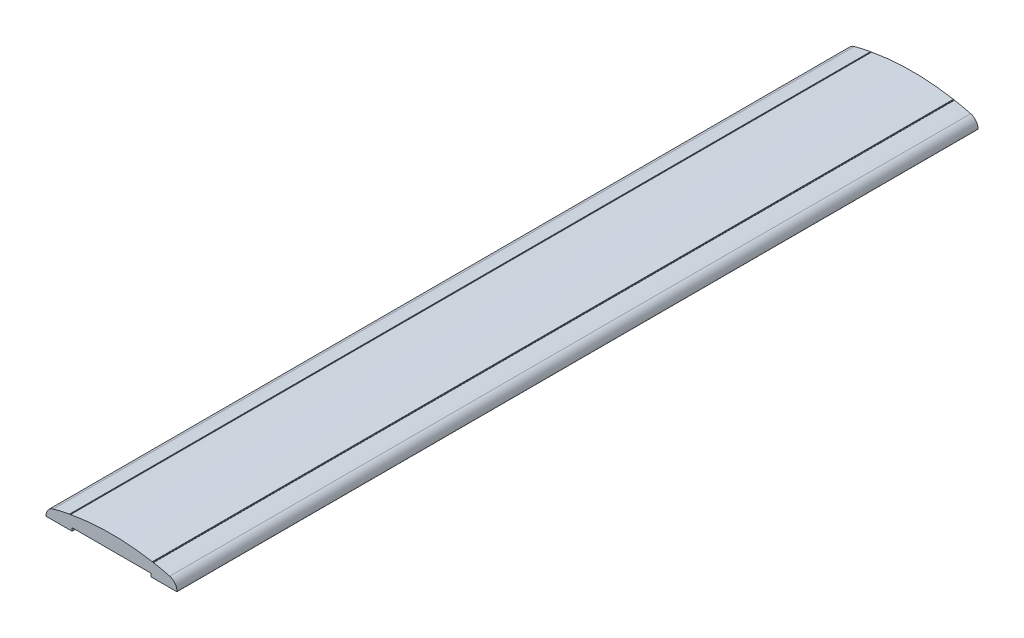
SolidWorks part; units mm, degrees
material "6063-T5"
ref_plane "前视基准面" through (0, 0, 0) normal (0, 0, 1) x (1, 0, 0)
ref_plane "上视基准面" through (0, 0, 0) normal (0, 1, 0) x (1, 0, 0)
ref_plane "右视基准面" through (0, 0, 0) normal (1, 0, 0) x (0, 0, -1)
sketch "草图1" plane through (0, 0, 0) normal (0, 0, 1) x (1, 0, 0)
  line L0 (0, 0) -> (0, -2.6973) construction
  line L1 (0, 25) -> (44.8763, 25) construction
  line L6 (94, 0) -> (56.7, 0)
  line L9 (56.5, 0.2) -> (56.5, 4.5)
  line L10 (-56.7, 0) -> (-94, 0)
  line L15 (-56.5, 0.2) -> (-56.5, 4.5)
  line L16 (0, 0) -> (0, 77.1229) construction
  line L21 (-56.5, 4.5) -> (56.5, 4.5)
  arc A2 (-60.272, 19.3814) -> (-59.7007, 19.4869) centre (-60, 19.5081) ccw
  arc A3 (-83.5579, 14.2629) -> (-94, 0) centre (-80.0184, 0.7177) ccw
  arc A5 (83.5579, 14.2629) -> (94, 0) centre (80.0184, 0.7177) cw
  arc A8 (-59.2723, 19.5653) -> (-58.7008, 19.669) centre (-59, 19.6911) ccw
  arc A10 (59.2723, 19.5653) -> (58.7008, 19.669) centre (59, 19.6911) cw
  arc A11 (-60.3809, 19.4375) -> (-83.5579, 14.2629) centre (0, -305.5) ccw
  arc A12 (60.272, 19.3814) -> (59.7007, 19.4869) centre (60, 19.5081) cw
  arc A13 (58.6188, 19.76) -> (-58.6188, 19.76) centre (0, -305.5) ccw
  arc A17 (56.7, 0) -> (56.5, 0.2) centre (56.7, 0.2) cw
  arc A18 (-56.5, 0.2) -> (-56.7, 0) centre (-56.7, 0.2) cw
  arc A20 (59.619, 19.5782) -> (59.3811, 19.6217) centre (0, -305.5) ccw
  arc A22 (-59.3811, 19.6217) -> (-59.619, 19.5782) centre (0, -305.5) ccw
  arc A23 (-58.7008, 19.669) -> (-58.6188, 19.76) centre (-58.6011, 19.6616) cw
  arc A24 (-59.2723, 19.5653) -> (-59.3811, 19.6217) centre (-59.3631, 19.5234) ccw
  arc A25 (83.5579, 14.2629) -> (60.3809, 19.4375) centre (0, -305.5) ccw
  arc A26 (-59.7007, 19.4869) -> (-59.619, 19.5782) centre (-59.601, 19.4798) cw
  arc A27 (-60.272, 19.3814) -> (-60.3809, 19.4375) centre (-60.3626, 19.3392) ccw
  arc A28 (58.6188, 19.76) -> (58.7008, 19.669) centre (58.6011, 19.6616) cw
  arc A29 (59.3811, 19.6217) -> (59.2723, 19.5653) centre (59.3631, 19.5234) ccw
  arc A30 (59.7007, 19.4869) -> (59.619, 19.5782) centre (59.601, 19.4798) ccw
  arc A31 (60.3809, 19.4375) -> (60.272, 19.3814) centre (60.3626, 19.3392) ccw
  point P58 (56.5, 0)
  point P61 (-56.5, 0)
  point P64 (-58.7048, 19.7445)
  point P67 (-59.2952, 19.6374)
  point P71 (-59.705, 19.5624)
  point P74 (-60.295, 19.4535)
  point P78 (58.7048, 19.7445)
  point P81 (59.2952, 19.6374)
  point P84 (59.705, 19.5624)
  point P87 (60.295, 19.4535)
  dimension "D16" = 1
  dimension "D21" = 0.1
  dimension "D22" = 0.1
  dimension "D23" = 0.1
  dimension "D10" = 0.6
  dimension "D24" = 0.1
  dimension "D25" = 0.1
  dimension "D26" = 0.1
  dimension "D27" = 0.1
  dimension "D28" = 0.1
extrude "凸台-拉伸1" add sketch "草图1" along normal mid plane 1150
fillet "圆角1" radius 0.3 2 edges at (-94, 0, 0) (94, 0, 0)
